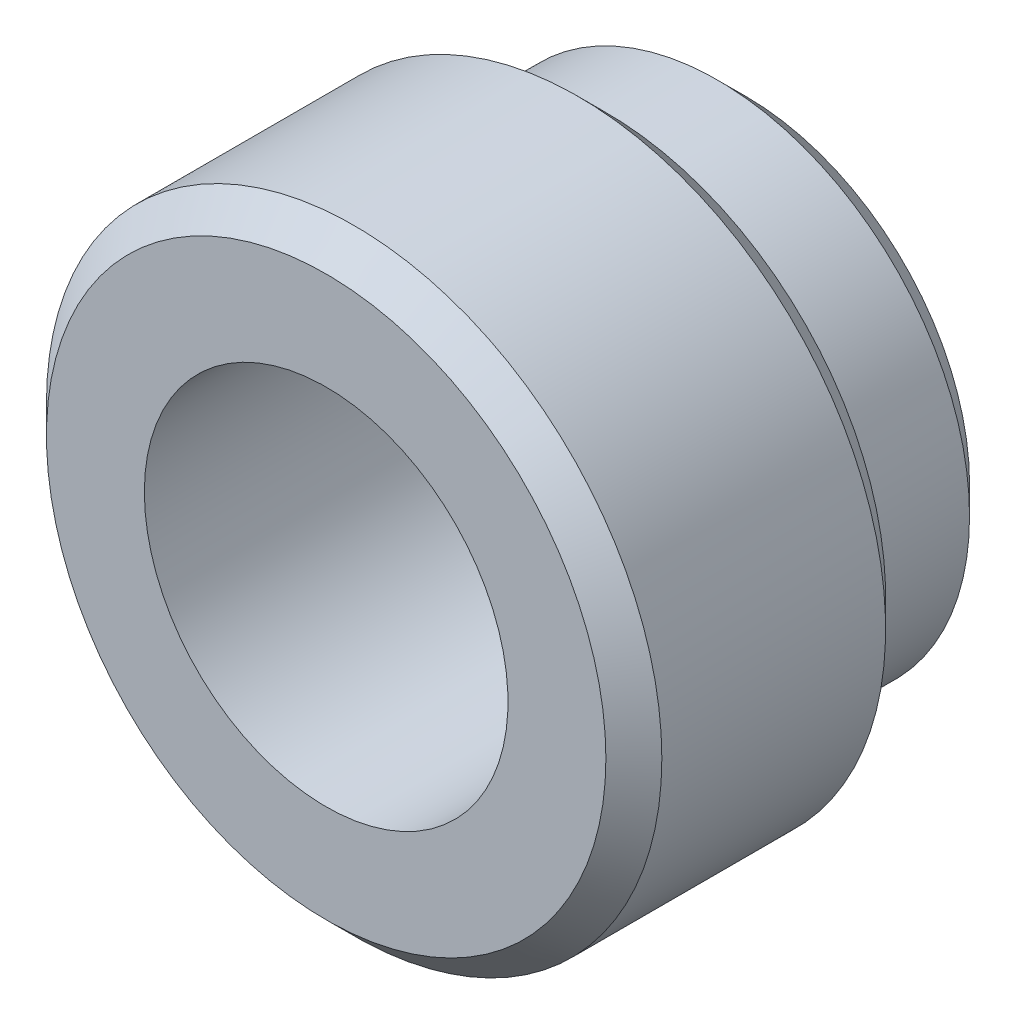
from build123d import *

# Parameters (mm, degrees)
SKETCH1_R           = 11
BOSS_EXTRUDE1_DEPTH = 15
SKETCH2_R           = 11
SKETCH2_R_2         = 9
CUT_EXTRUDE1_DEPTH  = 5
SKETCH3_R           = 6.5
CUT_EXTRUDE2_DEPTH  = 22.610182785
CHAMFER1_SIZE       = 1


with BuildPart() as part:
    # Sketch1 → Boss-Extrude1 (new body)
    with BuildSketch(Plane.XY):
        Circle(SKETCH1_R)
    extrude(amount=BOSS_EXTRUDE1_DEPTH)

    # Sketch2 → Cut-Extrude1 (cut)
    with BuildSketch(Plane(origin=(0, 0, 0), x_dir=(-1, 0, 0), z_dir=(0, 0, -1))):
        Circle(SKETCH2_R)
        Circle(SKETCH2_R_2, mode=Mode.SUBTRACT)
    extrude(amount=-CUT_EXTRUDE1_DEPTH, mode=Mode.SUBTRACT)

    # Sketch3 → Cut-Extrude2 (cut, through all)
    with BuildSketch(Plane(origin=(0, 0, 0), x_dir=(-1, 0, 0), z_dir=(0, 0, -1))):
        Circle(SKETCH3_R)
    extrude(amount=-CUT_EXTRUDE2_DEPTH, mode=Mode.SUBTRACT)

    # Chamfer1
    chamfer1_edges = [part.edges().sort_by_distance(p)[0] for p in [
        (-11, 0, 15),
        (-11, 0, 5),
        (9, 0, 0),
    ]]
    chamfer(chamfer1_edges, length=CHAMFER1_SIZE)


solid = part.part
